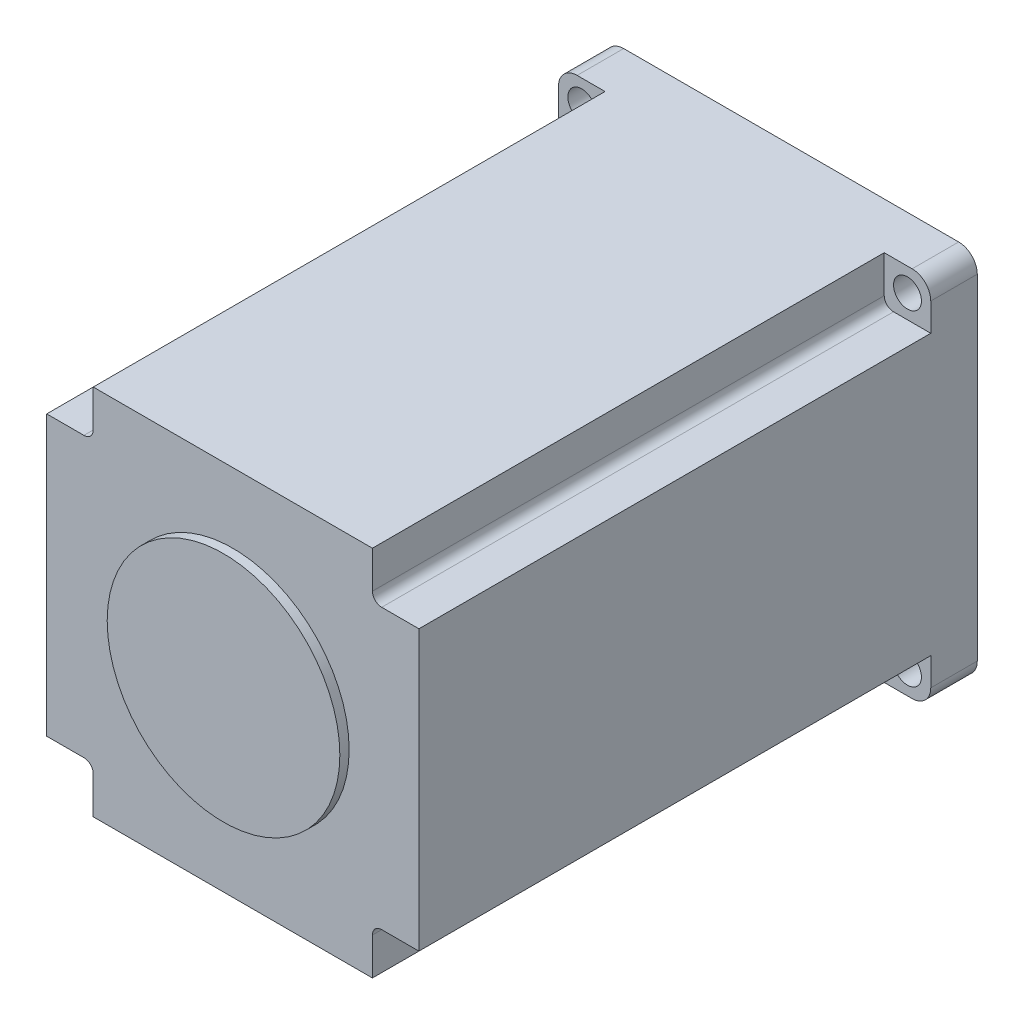
SolidWorks part; units mm, degrees
ref_plane "Front Plane" through (0, 0, 0) normal (0, 0, 1) x (1, 0, 0)
ref_plane "Top Plane" through (0, 0, 0) normal (0, 1, 0) x (1, 0, 0)
ref_plane "Right Plane" through (0, 0, 0) normal (1, 0, 0) x (0, 0, -1)
other "Configuration Table"
sketch "Sketch1" plane through (0, 0, 0) normal (0, 0, 1) x (1, 0, 0)
  line L1 (-20, 20) -> (20, 20)
  line L2 (-20, 20) -> (-20, -20)
  line L3 (-20, -20) -> (20, -20)
  line L4 (20, 20) -> (20, -20)
  line L5 (-20, 20) -> (20, -20) construction
  line L6 (-20, -20) -> (20, 20) construction
  point P0 (0, 0)
  dimension "D1" = 40
  dimension "D2" = 40
extrude "Boss-Extrude1" add sketch "Sketch1" along normal mid plane 60
sketch "Sketch2" plane through (0, 0, 30) normal (0, 0, 1) x (1, 0, 0)
  line L1 (-20, 20) -> (-15, 20)
  line L2 (-20, 20) -> (-20, 15)
  line L3 (-20, 15) -> (-15, 15)
  line L4 (-15, 20) -> (-15, 15)
  line L5 (20, 20) -> (15, 20)
  line L6 (20, 20) -> (20, 15)
  line L7 (20, 15) -> (15, 15)
  line L8 (15, 20) -> (15, 15)
  line L9 (20, -20) -> (15, -20)
  line L10 (20, -20) -> (20, -15)
  line L11 (20, -15) -> (15, -15)
  line L12 (15, -20) -> (15, -15)
  line L13 (-20, -20) -> (-15, -20)
  line L14 (-20, -20) -> (-20, -15)
  line L15 (-20, -15) -> (-15, -15)
  line L16 (-15, -20) -> (-15, -15)
  dimension "D1" = 5
  dimension "D2" = 5
  dimension "D3" = 5
  dimension "D4" = 5
  dimension "D5" = 5
extrude "Cut-Extrude1" cut sketch "Sketch2" against normal blind 55
sketch "Sketch3" plane through (0, 0, -25) normal (0, 0, 1) x (1, 0, 0)
  line L0 (-17.5, 20) -> (-17.5, 17.5) construction
  line L1 (-15, 20) -> (-20, 20) construction
  line L2 (-20, 17.5) -> (-17.5, 17.5) construction
  line L3 (-20, 20) -> (-20, 15) construction
  line L4 (0, 0) -> (0, 20) construction
  line L5 (15, 20) -> (-15, 20) construction
  line L6 (0, 0) -> (20, 0) construction
  line L7 (20, -15) -> (20, 15) construction
  circle A0 centre (-17.5, 17.5) radius 1.5
  circle A1 centre (17.5, 17.5) radius 1.5
  circle A2 centre (17.5, -17.5) radius 1.5
  circle A3 centre (-17.5, -17.5) radius 1.5
  dimension "D1" = 3
extrude "Cut-Extrude2" cut sketch "Sketch3" against normal blind 55
fillet "Fillet1" radius 2 4 edges at (-20, -20, -27.5) (20, -20, -27.5) (20, 20, -27.5) (-20, 20, -27.5)
sketch "Sketch4" plane through (0, 0, 30) normal (0, 0, 1) x (1, 0, 0)
  circle A0 centre (0, 0) radius 12.5
  dimension "D1" = 25
extrude "Boss-Extrude2" add sketch "Sketch4" along normal mid plane 2 contours A0
fillet "Fillet2" radius 1 4 edges at (-15, -15, 2.5) (15, -15, 2.5) (15, 15, 2.5) (-15, 15, 2.5)
sketch "Sketch5" plane through (0, 0, -30) normal (0, 0, -1) x (-1, 0, 0)
  circle A0 centre (0, 0) radius 5
  dimension "D1" = 10
extrude "Boss-Extrude3" add sketch "Sketch5" along normal blind 15
